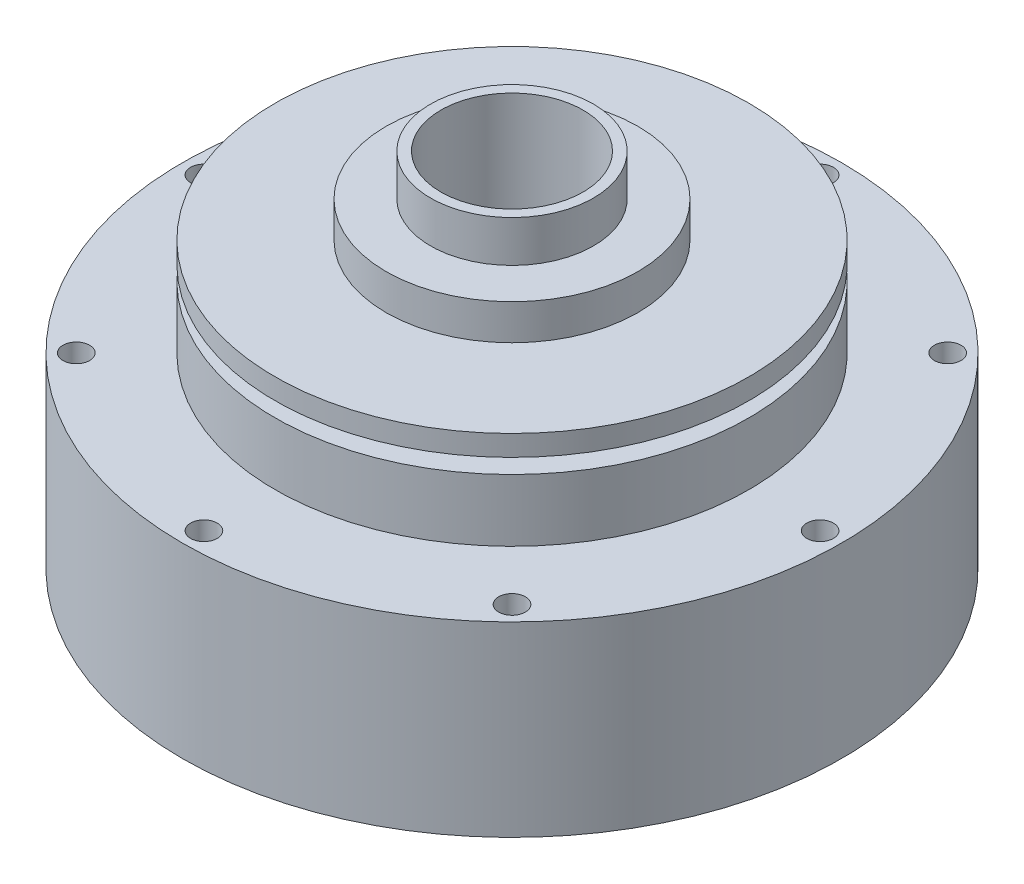
SolidWorks part; units mm, degrees
material "标准件"
ref_plane "前视基准面" through (0, 0, 0) normal (0, 0, 1) x (1, 0, 0)
ref_plane "上视基准面" through (0, 0, 0) normal (0, 1, 0) x (1, 0, 0)
ref_plane "右视基准面" through (0, 0, 0) normal (1, 0, 0) x (0, 0, -1)
sketch "草图1" plane through (0, 0, 0) normal (0, 0, 1) x (1, 0, 0)
  line L0 (0, 0) -> (0, 127) construction
  line L1 (0, 0) -> (87.5, 0)
  line L2 (87.5, 0) -> (87.5, 5)
  line L3 (87.5, 5) -> (111.25, 5)
  line L4 (111.25, 5) -> (111.25, 68)
  line L5 (111.25, 68) -> (80, 68)
  line L6 (80, 68) -> (80, 101)
  line L7 (80, 101) -> (42.5, 101)
  line L8 (42.5, 101) -> (42.5, 113)
  line L9 (42.5, 113) -> (27.5, 113)
  line L10 (27.5, 113) -> (27.5, 127)
  line L11 (27.5, 127) -> (0, 127)
  line L12 (0, 0) -> (0, 127)
  dimension "D1" = 222.5
  dimension "D2" = 63
  dimension "D3" = 160
  dimension "D4" = 85
  dimension "D5" = 55
  dimension "D6" = 5
  dimension "D7" = 87.5
  dimension "D8" = 33
  dimension "D9" = 12
  dimension "D10" = 127
revolve "旋转1" add sketch "草图1" angle 360 about L0
sketch "草图2" plane through (0, 127, 0) normal (0, 1, 0) x (1, 0, 0)
  circle A0 centre (0, 0) radius 24
  dimension "D1" = 48
extrude "切除-拉伸1" cut sketch "草图2" against normal through all
hole_wizard "M8 间隙孔1" positions "草图3" profile "草图4" hole size "M8" standard "ISO" end condition through all
sketch "草图3" plane through (0, 68, 0) normal (0, 1, 0) x (1, 0, 0)
  line L0 (0, 0) -> (0, 111.25) construction
  line L2 (0, 0) -> (0, 104) construction
  circle A0 centre (0, 0) radius 111.25 construction
  point P0 (0, 104)
  point P14 (73.5391, 73.5391)
  point P15 (104, 0)
  point P16 (73.5391, -73.5391)
  point P17 (0, -104)
  point P18 (-73.5391, -73.5391)
  point P19 (-104, 0)
  point P20 (-73.5391, 73.5391)
  dimension "D3" = 104
  dimension "D2" = 8
sketch "草图4" plane through (0, 68, -104) normal (1, 0, 0) x (0, 0, 1)
  line L0 (0, 0) -> (0, 68)
  line L1 (0, 68) -> (4.5, 68)
  line L2 (4.5, 68) -> (4.5, 0)
  line L5 (4.5, 0) -> (0, 0)
  line L11 (0, -6.35) -> (0, 107.95) construction
  dimension "通孔孔直径" = 9
  dimension "通孔孔深度" = 68
ref_plane "基准面1" through (0, 97.5, 0) normal (0, 1, 0) x (1, 0, 0)
sketch "草图5" plane through (0, 97.5, 0) normal (0, 1, 0) x (1, 0, 0)
  circle A0 centre (0, 0) radius 78
  dimension "D1" = 156
sketch "草图7" plane through (0, 0, 0) normal (0, 0, 1) x (1, 0, 0)
  line L0 (0, 0) -> (0, 127) construction
  line L1 (-87.5, 0) -> (87.5, 0) construction
  line L2 (27.5, 127) -> (-27.5, 127) construction
  line L3 (80, 68) -> (80, 101) construction
  line L4 (70, 94) -> (80, 94)
  line L5 (70, 94) -> (70, 89)
  line L6 (70, 89) -> (80, 89)
  line L7 (80, 94) -> (80, 89)
  line L8 (80, 101) -> (-80, 101) construction
  dimension "D1" = 5
  dimension "D2" = 7
  dimension "D3" = 10
revolve "切除-旋转1" cut sketch "草图7" angle 360 about L0
hole_wizard "M10 螺纹孔1" positions "草图8" profile "草图9" tap size "M10" standard "ISO"
sketch "草图8" plane through (0, 0, 0) normal (0, -1, 0) x (-1, 0, 0)
  line L0 (0, 67) -> (0, 0)
  line L2 (0, 0) -> (0, 67) construction
  point P0 (0, 67)
  point P12 (47.3762, 47.3762)
  point P13 (67, 0)
  point P14 (47.3762, -47.3762)
  point P15 (0, -67)
  point P16 (-47.3762, -47.3762)
  point P17 (-67, 0)
  point P18 (-47.3762, 47.3762)
  dimension "D3" = 67
  dimension "D2" = 8
sketch "草图9" plane through (0, 0, -67) normal (1, 0, 0) x (0, 0, -1)
  line L0 (0, 0) -> (0, 27.0537)
  line L1 (0, 27.0537) -> (4.25, 24.5)
  line L2 (4.25, 24.5) -> (4.25, 0)
  line L5 (4.25, 0) -> (0, 0)
  line L10 (0, 27.0537) -> (-4.25, 24.5) construction
  line L11 (0, -6.35) -> (0, 107.95) construction
  dimension "螺纹孔钻头直径" = 8.5
  dimension "螺纹孔钻头深度" = 24.5
  dimension "导头角度" = 118
cosmetic thread "孔螺蚊线1" parameters "D1"=20, "D2"=10
cosmetic thread "孔螺蚊线2" parameters "D1"=20, "D2"=10
cosmetic thread "孔螺蚊线3" parameters "D1"=20, "D2"=10
cosmetic thread "孔螺蚊线4" parameters "D1"=20, "D2"=10
cosmetic thread "孔螺蚊线5" parameters "D1"=20, "D2"=10
cosmetic thread "孔螺蚊线6" parameters "D1"=20, "D2"=10
cosmetic thread "孔螺蚊线7" parameters "D1"=20, "D2"=10
cosmetic thread "孔螺蚊线8" parameters "D1"=20, "D2"=10
